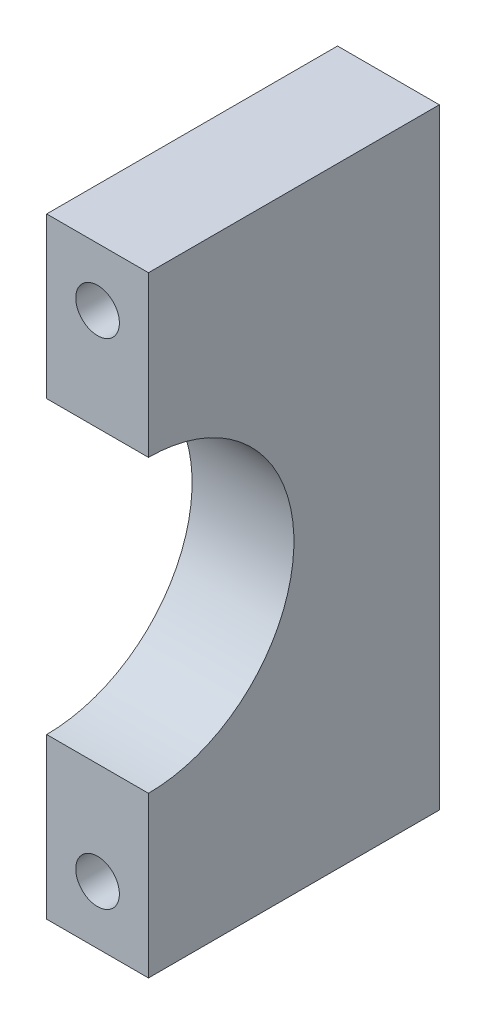
from build123d import *

# Parameters (mm, degrees)
SKETCH2_W           = 3.5
SKETCH2_H           = 10
BOSS_EXTRUDE1_DEPTH = 10.5
SKETCH3_R           = 0.75
CUT_EXTRUDE1_DEPTH  = 15.91643389
SKETCH4_R           = 5
CUT_EXTRUDE2_DEPTH  = 18.073371079


with BuildPart() as part:
    # Sketch2 → Boss-Extrude1 (new, symmetric)
    with BuildSketch(Plane(origin=(0, 0, 0), x_dir=(1, 0, 0), z_dir=(0, 1, 0))):
        with Locations((-1.75, 8)):
            Rectangle(SKETCH2_W, SKETCH2_H)
    extrude(amount=BOSS_EXTRUDE1_DEPTH, both=True)

    # Sketch3 → Cut-Extrude1 (cut, through all)
    with BuildSketch(Plane(origin=(0, 0, -13), x_dir=(-1, 0, 0), z_dir=(0, 0, -1))):
        with Locations((1.75, -8.5)):
            Circle(SKETCH3_R)
        with Locations(Location((1.75, 8.5, 0), (0, 0, 180))):
            Circle(SKETCH3_R)
    extrude(amount=-CUT_EXTRUDE1_DEPTH, mode=Mode.SUBTRACT)

    # Sketch4 → Cut-Extrude2 (cut, through all)
    with BuildSketch(Plane.ZY.offset(3.5)):
        with Locations((-3, 0)):
            Circle(SKETCH4_R)
    extrude(amount=-CUT_EXTRUDE2_DEPTH, mode=Mode.SUBTRACT)


solid = part.part
